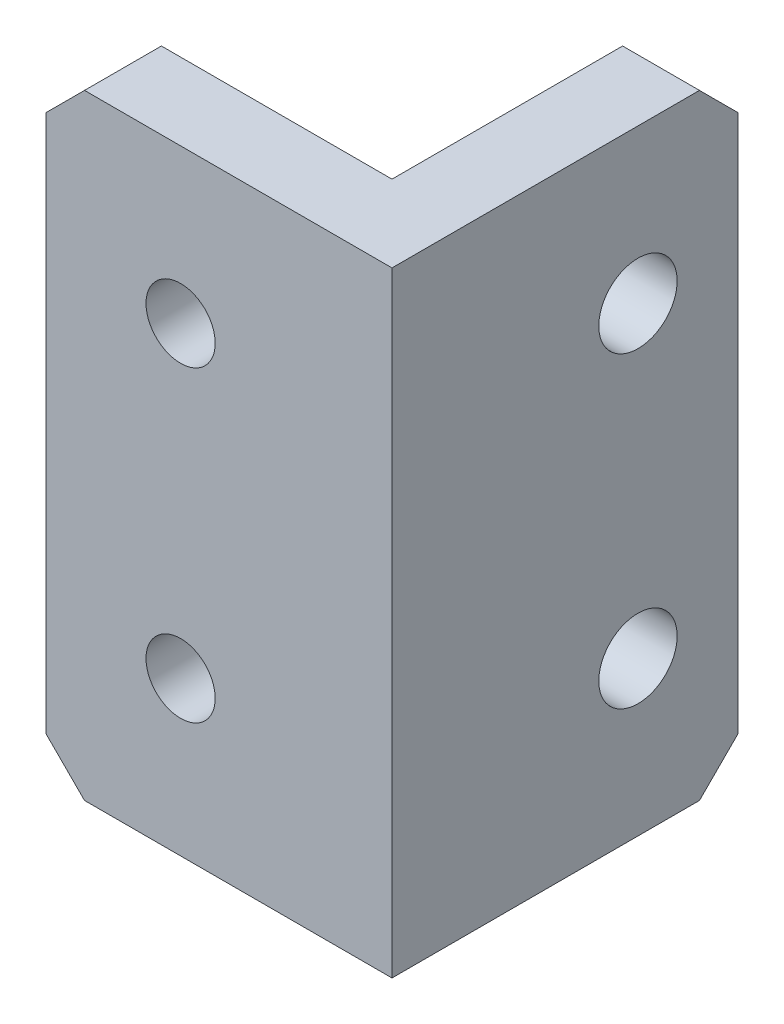
from build123d import *

# Parameters (mm, degrees)
EXTRUDE_1_DEPTH        = 80
CHAMFER_1_SIZE         = 5
HOLE_WIZARD_M8_1_D     = 9
HOLE_WIZARD_M8_1_DEPTH = 15
HOLE_WIZARD_M8_1_TIP   = 2.703872786
HOLE_WIZARD_M12_1_D    = 10.2
PATTERN_LINEAR_1_COUNT = 2
PATTERN_LINEAR_1_PITCH = 40


with BuildPart() as part:
    # 草图1 → 凸台-拉伸1 (new body)
    with BuildSketch(Plane(origin=(0, 0, 0), x_dir=(1, 0, 0), z_dir=(0, 1, 0))):
        Polygon((-22.5, -12.5), (12.5, -12.5), (12.5, 22.5), (22.5, 22.5), (22.5, -22.5), (-22.5, -22.5), align=None)
    extrude(amount=EXTRUDE_1_DEPTH)

    # 倒角1
    chamfer_1_edges = [part.edges().sort_by_distance(p)[0] for p in [
        (-22.5, 80, 17.5),
        (-22.5, 0, 17.5),
        (17.5, 80, -22.5),
        (17.5, 0, -22.5),
    ]]
    chamfer(chamfer_1_edges, length=CHAMFER_1_SIZE)

    # M8 间隙孔1
    with Locations(Plane(origin=(-5, 60, 12.5), x_dir=(-1, 0, 0), z_dir=(0, 0, -1))):
        with Locations((0, 0), (0, -40)):
            Hole(HOLE_WIZARD_M8_1_D / 2, depth=HOLE_WIZARD_M8_1_DEPTH)
            with Locations((0, 0, -(HOLE_WIZARD_M8_1_DEPTH + HOLE_WIZARD_M8_1_TIP / 2))):  # 118° drill point
                Cone(0, HOLE_WIZARD_M8_1_D / 2, HOLE_WIZARD_M8_1_TIP, mode=Mode.SUBTRACT)

    # M12 螺纹孔1 (through all)
    with Locations(Plane(origin=(12.5, 60, -9.5), x_dir=(0, 0, -1), z_dir=(-1, 0, 0))):
        with Locations((0, 0)):
            hole_wizard_m12_1 = Hole(HOLE_WIZARD_M12_1_D / 2)

    # 阵列(线性)1: M12 螺纹孔1 ×2
    with Locations(*[(0, -i * PATTERN_LINEAR_1_PITCH, 0) for i in range(1, PATTERN_LINEAR_1_COUNT)]):
        add(hole_wizard_m12_1, mode=Mode.SUBTRACT)


solid = part.part
